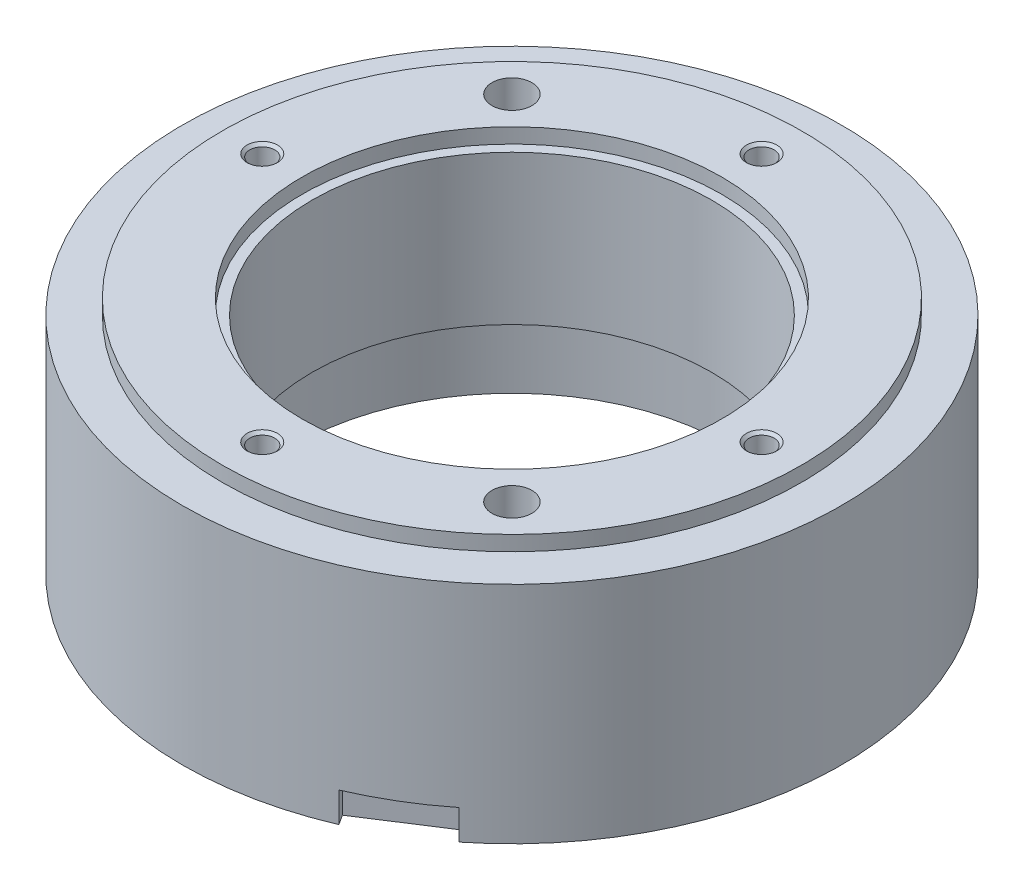
from build123d import *

# Parameters (mm, degrees)
SKETCH1_R                     = 33
BOSS_EXTRUDE1_DEPTH           = 22.5
SKETCH2_R                     = 29
BOSS_EXTRUDE2_DEPTH           = 1.5
SKETCH3_R                     = 20
CUT_EXTRUDE1_DEPTH            = 58.5
M3_TAPPED_HOLE1_D             = 2.5
M3_TAPPED_HOLE1_DEPTH         = 7.5
M3_TAPPED_HOLE1_CSINK_D       = 3.05
M3_TAPPED_HOLE1_CSINK_ANGLE   = 90
M3_TAPPED_HOLE1_TIP           = 0.751075774
SKETCH7_R                     = 2
CUT_EXTRUDE2_DEPTH            = 5
SKETCH8_R                     = 21
CUT_EXTRUDE3_DEPTH            = 1.5
SKETCH9_R                     = 29
CUT_EXTRUDE4_DEPTH            = 0.36
SKETCH10_R                    = 21.75
CUT_EXTRUDE5_DEPTH            = 7.2
M1_6_TAPPED_HOLE1_D           = 1.25
M1_6_TAPPED_HOLE1_DEPTH       = 4.25
M1_6_TAPPED_HOLE1_CSINK_D     = 1.65
M1_6_TAPPED_HOLE1_CSINK_ANGLE = 90
M1_6_TAPPED_HOLE1_TIP         = 0.375537887
CUT_EXTRUDE6_DEPTH            = 3


with BuildPart() as part:
    # Sketch1 → Boss-Extrude1 (new body)
    with BuildSketch(Plane(origin=(0, 0, 0), x_dir=(1, 0, 0), z_dir=(0, 1, 0))):
        with Locations(Location((0, 0, 0), (0, 0, 90))):
            Circle(SKETCH1_R)
    extrude(amount=BOSS_EXTRUDE1_DEPTH)

    # Sketch2 → Boss-Extrude2 (add)
    with BuildSketch(Plane(origin=(0, 22.5, 0), x_dir=(1, 0, 0), z_dir=(0, 1, 0))):
        with Locations(Location((0, 0, 0), (0, 0, 270))):
            Circle(SKETCH2_R)
    extrude(amount=BOSS_EXTRUDE2_DEPTH)

    # Sketch3 → Cut-Extrude1 (cut)
    with BuildSketch(Plane(origin=(0, 24, 0), x_dir=(1, 0, 0), z_dir=(0, 1, 0))):
        with Locations(Location((0, 0, 0), (0, 0, 270))):
            Circle(SKETCH3_R)
    extrude(amount=-CUT_EXTRUDE1_DEPTH, mode=Mode.SUBTRACT)

    # M3 Tapped Hole1
    with Locations(Plane(origin=(0, 24, 0), x_dir=(1, 0, 0), z_dir=(0, 1, 0))):
        with Locations((25, 0), (0, 25), (-25, 0), (0, -25)):
            CounterSinkHole(M3_TAPPED_HOLE1_D / 2, M3_TAPPED_HOLE1_CSINK_D / 2, depth=M3_TAPPED_HOLE1_DEPTH, counter_sink_angle=M3_TAPPED_HOLE1_CSINK_ANGLE)
            with Locations((0, 0, -(M3_TAPPED_HOLE1_DEPTH + M3_TAPPED_HOLE1_TIP / 2))):  # 118° drill point
                Cone(0, M3_TAPPED_HOLE1_D / 2, M3_TAPPED_HOLE1_TIP, mode=Mode.SUBTRACT)

    # Sketch7 → Cut-Extrude2 (cut)
    with BuildSketch(Plane(origin=(0, 24, 0), x_dir=(1, 0, 0), z_dir=(0, 1, 0))):
        with Locations(Location((-17.67766953, 17.67766953, 0), (0, 0, 270))):
            Circle(SKETCH7_R)
        with Locations(Location((17.67766953, -17.67766953, 0), (0, 0, 270))):
            Circle(SKETCH7_R)
    extrude(amount=-CUT_EXTRUDE2_DEPTH, mode=Mode.SUBTRACT)

    # Sketch8 → Cut-Extrude3 (cut)
    with BuildSketch(Plane(origin=(0, 24, 0), x_dir=(1, 0, 0), z_dir=(0, 1, 0))):
        with Locations(Location((0, 0, 0), (0, 0, 270))):
            Circle(SKETCH8_R)
    extrude(amount=-CUT_EXTRUDE3_DEPTH, mode=Mode.SUBTRACT)

    # Sketch9 → Cut-Extrude4 (cut)
    with BuildSketch(Plane.XZ):
        with Locations(Location((0, 0, 0), (0, 0, 90))):
            Circle(SKETCH9_R)
    extrude(amount=-CUT_EXTRUDE4_DEPTH, mode=Mode.SUBTRACT)

    # Sketch10 → Cut-Extrude5 (cut)
    with BuildSketch(Plane.XZ.offset(-0.36)):
        with Locations(Location((0, 0, 0), (0, 0, 270))):
            Circle(SKETCH10_R)
    extrude(amount=-CUT_EXTRUDE5_DEPTH, mode=Mode.SUBTRACT)

    # M1.6 Tapped Hole1
    with Locations(Plane(origin=(0, 0, 0), x_dir=(-1, 0, 0), z_dir=(0, -1, 0))):
        with Locations((0, 0), (0, 31), (26.846787517, 15.5), (26.846787517, -15.5), (0, -31), (-26.846787517, -15.5), (-26.846787517, 15.5)):
            CounterSinkHole(M1_6_TAPPED_HOLE1_D / 2, M1_6_TAPPED_HOLE1_CSINK_D / 2, depth=M1_6_TAPPED_HOLE1_DEPTH, counter_sink_angle=M1_6_TAPPED_HOLE1_CSINK_ANGLE)
            with Locations((0, 0, -(M1_6_TAPPED_HOLE1_DEPTH + M1_6_TAPPED_HOLE1_TIP / 2))):  # 118° drill point
                Cone(0, M1_6_TAPPED_HOLE1_D / 2, M1_6_TAPPED_HOLE1_TIP, mode=Mode.SUBTRACT)

    # Sketch15 → Cut-Extrude6 (cut)
    with BuildSketch(Plane.XZ):
        Polygon((19.632226772, 24.641961986), (12.362677286, 29.333923153), (15.170555531, 33.68434489), (22.766930333, 28.781441946), align=None)
    extrude(amount=-CUT_EXTRUDE6_DEPTH, mode=Mode.SUBTRACT)


solid = part.part
